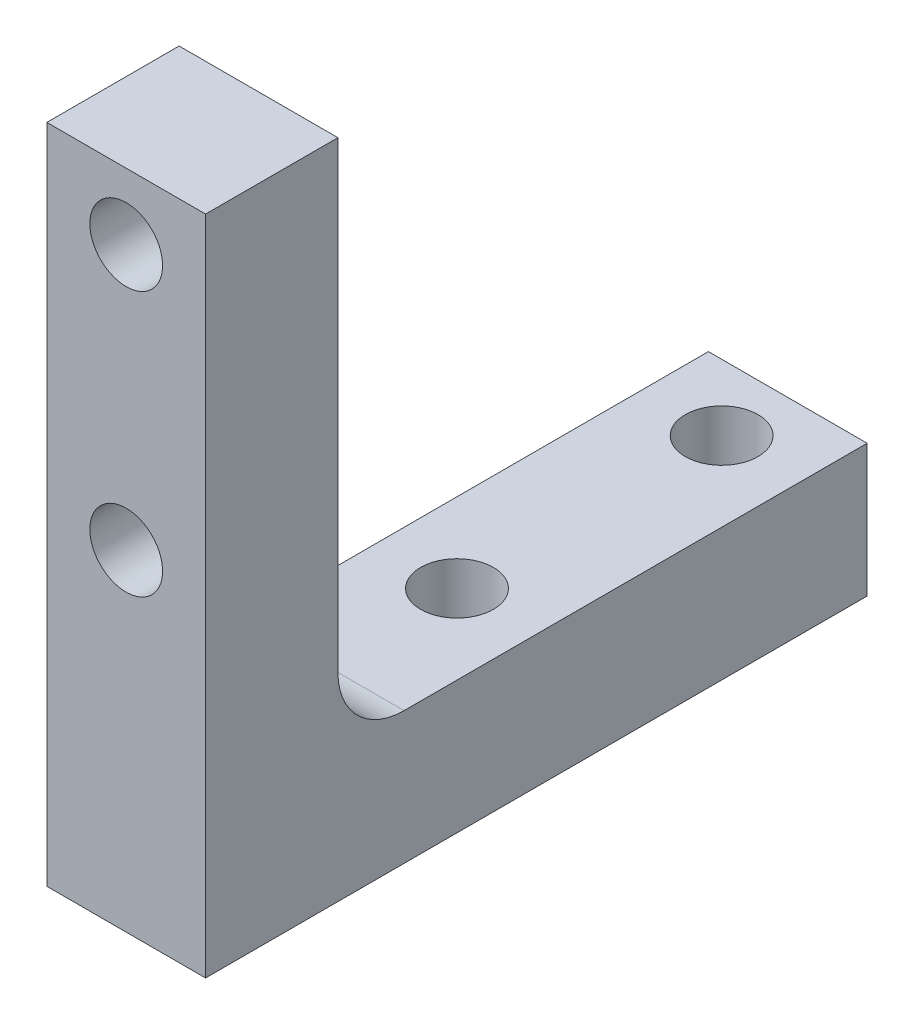
from build123d import *

# Parameters (mm, degrees)
BOSS_EXTRUDE1_DEPTH  = 12
FILLET1_R            = 5
M5_CLEARANCE_HOLE1_D = 5.5
M5_CLEARANCE_HOLE2_D = 5.5


with BuildPart() as part:
    # Sketch1 → Boss-Extrude1 (new body)
    with BuildSketch(Plane(origin=(0, 0, 0), x_dir=(0, 0, -1), z_dir=(1, 0, 0))):
        Polygon((0, 0), (0, 50), (10, 50), (10, 10), (50, 10), (50, 0), align=None)
    extrude(amount=BOSS_EXTRUDE1_DEPTH)

    # Fillet1
    fillet1_edges = [part.edges().sort_by_distance(p)[0] for p in [
        (6, 10, -10),
    ]]
    fillet(fillet1_edges, radius=FILLET1_R)

    # M5 Clearance Hole1 (through all)
    with Locations(Plane(origin=(0, 0, -10), x_dir=(-1, 0, 0), z_dir=(0, 0, -1))):
        with Locations((-6, 25), (-6, 45)):
            Hole(M5_CLEARANCE_HOLE1_D / 2)

    # M5 Clearance Hole2 (through all)
    with Locations(Plane(origin=(0, 10, 0), x_dir=(1, 0, 0), z_dir=(0, 1, 0))):
        with Locations((6, 45), (6, 25)):
            Hole(M5_CLEARANCE_HOLE2_D / 2)


solid = part.part
